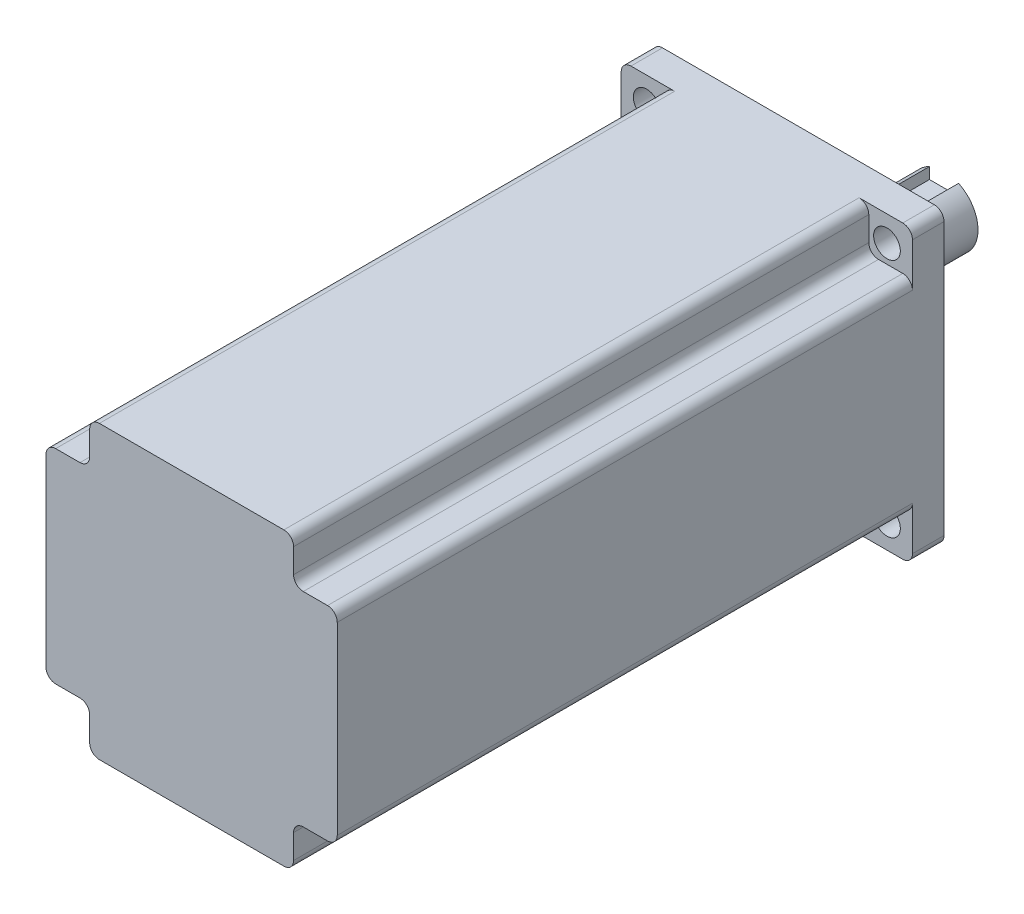
SolidWorks part; units mm, degrees
ref_plane "前视基准面" through (0, 0, 0) normal (0, 0, 1) x (1, 0, 0)
ref_plane "上视基准面" through (0, 0, 0) normal (0, 1, 0) x (1, 0, 0)
ref_plane "右视基准面" through (0, 0, 0) normal (1, 0, 0) x (0, 0, -1)
sketch "草图1" plane through (0, 0, 0) normal (0, 0, 1) x (1, 0, 0)
  line L1 (-30, 30) -> (30, 30)
  line L2 (-30, 30) -> (-30, -30)
  line L3 (-30, -30) -> (30, -30)
  line L4 (30, 30) -> (30, -30)
  line L5 (-30, 30) -> (30, -30) construction
  line L6 (-30, -30) -> (30, 30) construction
  point P0 (0, 0)
  dimension "D1" = 60
  dimension "D2" = 60
extrude "凸台-拉伸1" add sketch "草图1" along normal blind 125
sketch "草图2" plane through (0, 0, 0) normal (0, 0, -1) x (-1, 0, 0)
  circle A0 centre (0, 0) radius 25
  dimension "D1" = 50
extrude "凸台-拉伸2" add sketch "草图2" along normal blind 3
sketch "草图3" plane through (0, 0, -3) normal (0, 0, -1) x (-1, 0, 0)
  circle A0 centre (0, 0) radius 7
  dimension "D1" = 14
extrude "凸台-拉伸3" add sketch "草图3" along normal blind 27
ref_plane "基准面1" through (0, 7, 0) normal (0, 1, 0) x (1, 0, 0)
sketch "草图4" plane through (0, 7, 0) normal (0, 1, 0) x (1, 0, 0)
  line L0 (0, 34.3494) -> (0, -19.6368) construction
  line L1 (0, 30) -> (0, 7.5) construction
  line L2 (7, 30) -> (-7, 30) construction
  line L3 (3, 30) -> (3, 7.5)
  line L4 (-3, 30) -> (-3, 7.5)
  arc A0 (3, 30) -> (-3, 30) centre (0, 30) ccw
  arc A1 (-3, 7.5) -> (3, 7.5) centre (0, 7.5) ccw
  point P7 (0, 18.75)
  dimension "D1" = 22.5
  dimension "D2" = 6
extrude "切除-拉伸1" cut sketch "草图4" against normal blind 3 contours A0 L4 A1 L3
hole_wizard "M5 螺纹孔1" positions "草图6" profile "草图5" tap size "M5" standard "ISO"
sketch "草图6" plane through (0, 0, -30) normal (0, 0, -1) x (-1, 0, 0)
  point P0 (0, 0)
sketch "草图5" plane through (0, 0, -30) normal (1, 0, 0) x (0, 1, 0)
  line L0 (0, 0) -> (0, 7.2618)
  line L1 (0, 7.2618) -> (2.1, 6)
  line L2 (2.1, 6) -> (2.1, 0)
  line L5 (2.1, 0) -> (0, 0)
  line L10 (0, 7.2618) -> (-2.1, 6) construction
  line L11 (0, -6.35) -> (0, 107.95) construction
  dimension "螺纹孔钻头直径" = 4.2
  dimension "螺纹孔钻头深度" = 6
  dimension "导头角度" = 118
cosmetic thread "孔螺蚊线1" parameters "D1"=6, "D2"=5
hole_wizard "Ø4.5 (4.5) 直径孔1" positions "草图8" profile "草图7" hole size "Ø4.5" standard "GB"
sketch "草图8" plane through (0, 0, 0) normal (0, 0, -1) x (-1, 0, 0)
  line L0 (0, 0) -> (-24.7487, 24.7487) construction
  line L2 (0, 0) -> (24.7487, 24.7487) construction
  line L4 (0, 0) -> (0, 35) construction
  line L5 (-34.3548, 0) -> (40.4324, 0) construction
  circle A0 centre (0, 0) radius 35 construction
  point P7 (-24.7487, 24.7487)
  point P12 (24.7487, 24.7487)
  point P28 (24.7487, -24.7487)
  point P29 (-24.7487, -24.7487)
  dimension "D1" = 70
  dimension "D2" = 45
  dimension "D3" = 45
sketch "草图7" plane through (24.7487, 24.7487, 0) normal (1, 0, 0) x (0, 1, 0)
  line L0 (0, 0) -> (0, 11.6524)
  line L1 (0, 11.6524) -> (2.75, 10)
  line L2 (2.75, 10) -> (2.75, 0)
  line L5 (2.75, 0) -> (0, 0)
  line L10 (0, 11.6524) -> (-2.75, 10) construction
  line L11 (0, -6.35) -> (0, 107.95) construction
  dimension "孔直径" = 5.5
  dimension "孔深度" = 10
  dimension "导头角度" = 118
sketch "草图10" plane through (0, 0, 125) normal (0, 0, 1) x (1, 0, 0)
  line L1 (-30, 30) -> (-21, 30)
  line L2 (-30, 30) -> (-30, 21)
  line L3 (-30, 21) -> (-21, 21)
  line L4 (-21, 30) -> (-21, 21)
  dimension "D1" = 9
  dimension "D2" = 9
extrude "切除-拉伸2" cut sketch "草图10" against normal blind 118.5
mirror "镜向1" about plane through (0, 0, 0) normal (1, 0, 0) of "切除-拉伸2"
mirror "镜向2" about plane through (0, 0, 0) normal (0, 1, 0) of "镜向1", "切除-拉伸2"
fillet "圆角1" radius 2 16 edges at (-30, 30, 3.25) (-21, -21, 65.75) (-30, -30, 3.25) (21, -21, 65.75) (30, -30, 3.25) (30, 30, 3.25) (21, 21, 65.75) (-21, 21, 65.75) (21, -30, 65.75) (30, -21, 65.75) (-30, -21, 65.75) (-21, -30, 65.75) (-21, 30, 65.75) (-30, 21, 65.75) (30, 21, 65.75) (21, 30, 65.75)
